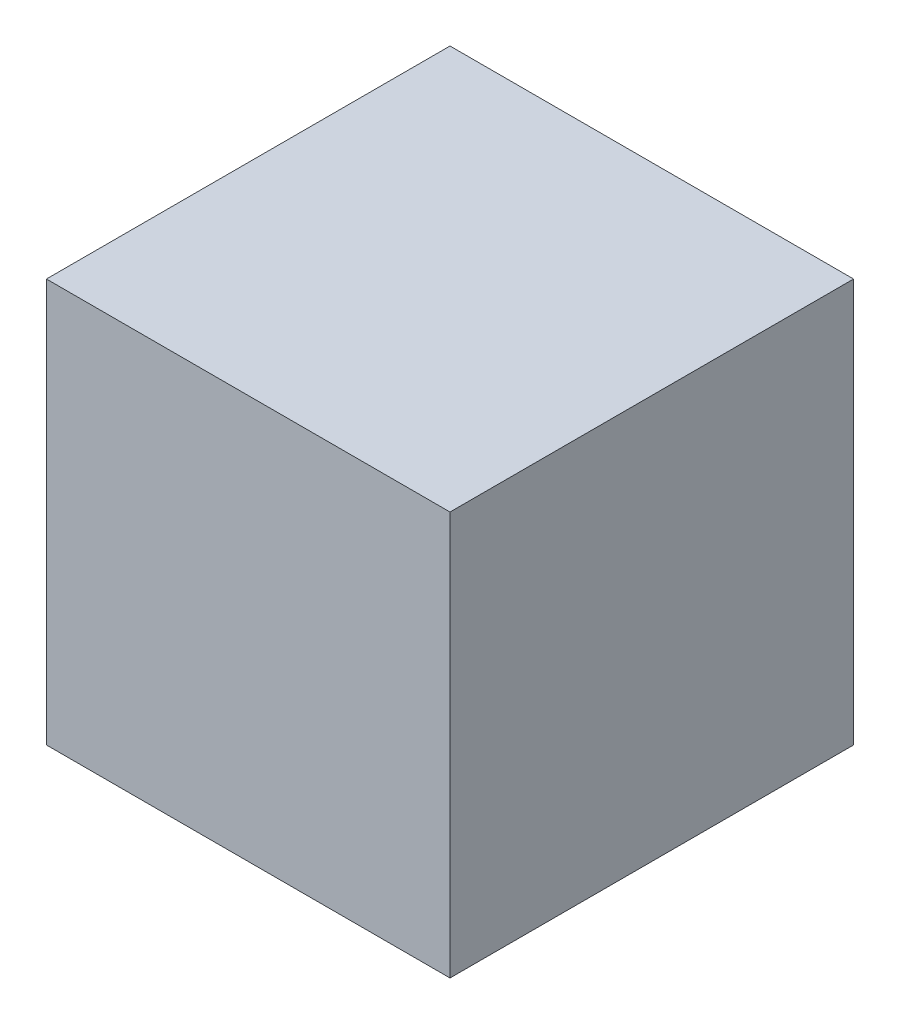
from build123d import *

# Parameters (mm, degrees)
SKETCH1_W           = 25
SKETCH1_H           = 25
BOSS_EXTRUDE1_DEPTH = 25


with BuildPart() as part:
    # Sketch1 → Boss-Extrude1 (new body)
    with BuildSketch(Plane(origin=(0, 0, 0), x_dir=(1, 0, 0), z_dir=(0, 1, 0))):
        Rectangle(SKETCH1_W, SKETCH1_H)
    extrude(amount=BOSS_EXTRUDE1_DEPTH)


solid = part.part
